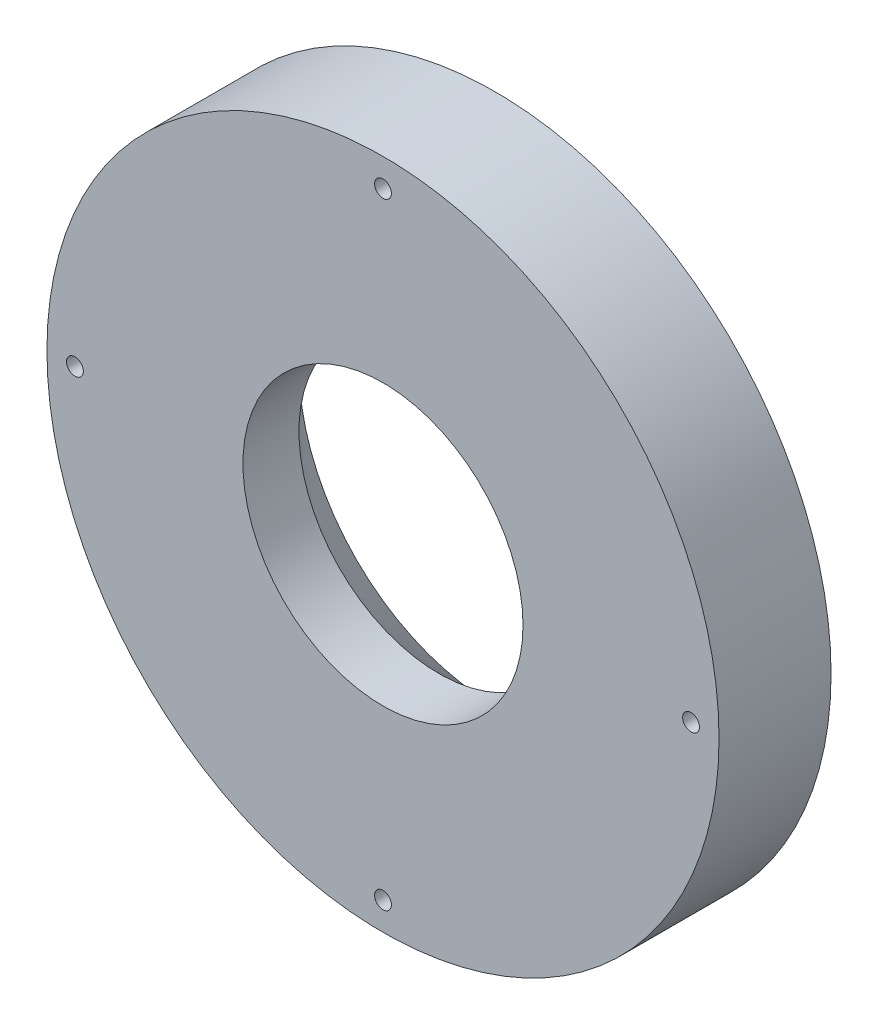
from build123d import *

# Parameters (mm, degrees)
SKETCH_1_R          = 60
SKETCH_1_R_2        = 25
EXTRUDE_1_DEPTH     = 20
CHAMFER_1_SIZE      = 10
SKETCH_2_R          = 1.5
CUT_EXTRUDE_1_DEPTH = 27


with BuildPart() as part:
    # 草图1 → 凸台-拉伸1 (new body)
    with BuildSketch(Plane.XY):
        Circle(SKETCH_1_R)
        Circle(SKETCH_1_R_2, mode=Mode.SUBTRACT)
    extrude(amount=EXTRUDE_1_DEPTH)

    # 倒角1
    chamfer_1_edges = [part.edges().sort_by_distance(p)[0] for p in [
        (-25, 0, 0),
    ]]
    chamfer(chamfer_1_edges, length=CHAMFER_1_SIZE)

    # 草图2 → 切除-拉伸1 (cut)
    with BuildSketch(Plane.XY.offset(20)):
        with Locations((0, 55)):
            Circle(SKETCH_2_R)
        with Locations((55, 0)):
            Circle(SKETCH_2_R)
        with Locations((0, -55)):
            Circle(SKETCH_2_R)
        with Locations((-55, 0)):
            Circle(SKETCH_2_R)
    extrude(amount=-CUT_EXTRUDE_1_DEPTH, mode=Mode.SUBTRACT)


solid = part.part
